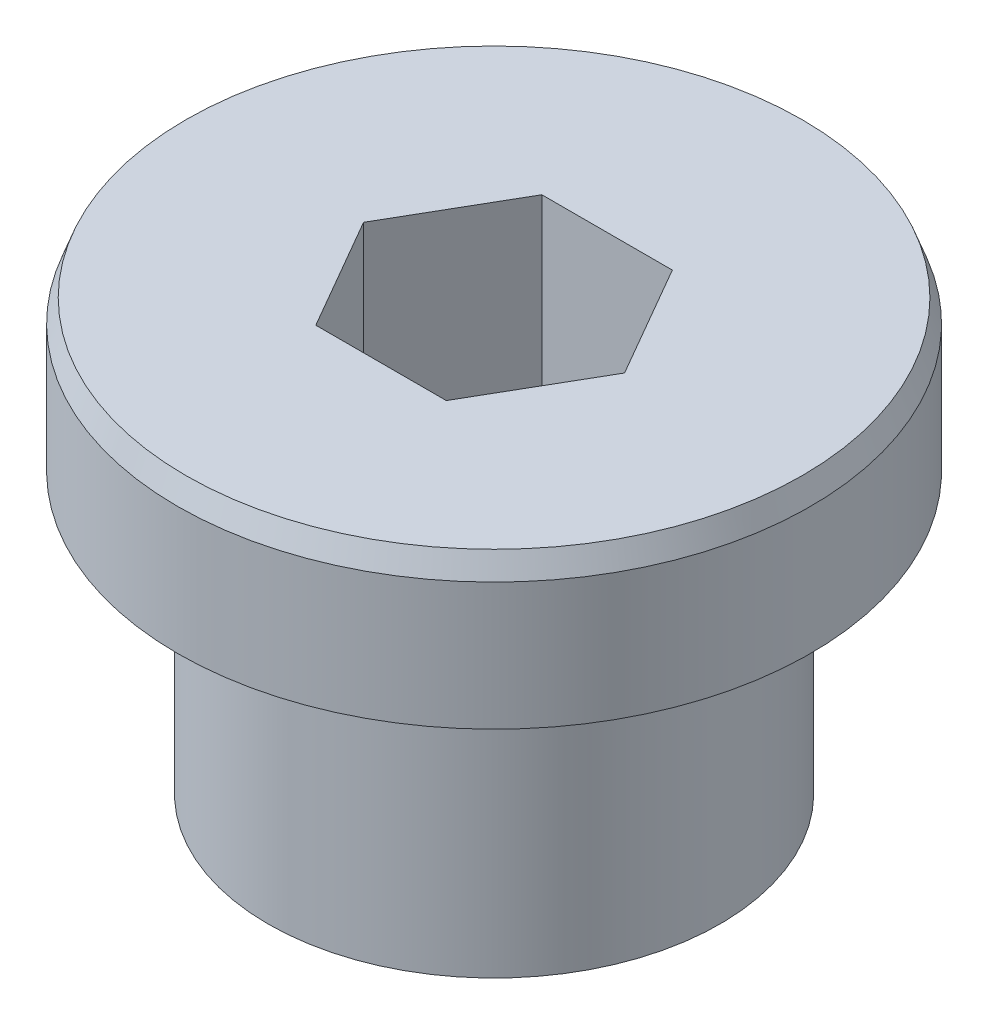
from build123d import *
from OCP.BRepFilletAPI import BRepFilletAPI_MakeChamfer

# Parameters (mm, degrees)
SKETCH1_R           = 5
BOSS_EXTRUDE1_DEPTH = 6
SKETCH3_R           = 7
BOSS_EXTRUDE2_DEPTH = 3.5
CUT_EXTRUDE1_DEPTH  = 5
CHAMFER1_SIZE       = 0.5
CHAMFER1_SIZE2      = 0.181985117


with BuildPart() as part:
    # Sketch1 → Boss-Extrude1 (new body)
    with BuildSketch(Plane(origin=(0, 0, 0), x_dir=(1, 0, 0), z_dir=(0, 1, 0))):
        with Locations(Location((0, 0, 0), (0, 0, 270))):
            Circle(SKETCH1_R)
    extrude(amount=BOSS_EXTRUDE1_DEPTH)

    # Sketch3 → Boss-Extrude2 (add)
    with BuildSketch(Plane(origin=(0, 6, 0), x_dir=(1, 0, 0), z_dir=(0, 1, 0))):
        with Locations(Location((0, 0, 0), (0, 0, 270))):
            Circle(SKETCH3_R)
    extrude(amount=BOSS_EXTRUDE2_DEPTH)

    # Sketch4 → Cut-Extrude1 (cut)
    with BuildSketch(Plane(origin=(0, 9.5, 0), x_dir=(1, 0, 0), z_dir=(0, 1, 0))):
        Polygon((-2.886751346, 0), (-1.443375673, -2.5), (1.443375673, -2.5), (2.886751346, 0), (1.443375673, 2.5), (-1.443375673, 2.5), align=None)
    extrude(amount=-CUT_EXTRUDE1_DEPTH, mode=Mode.SUBTRACT)

    # Chamfer1: one chamfer whose edges measure the first distance from different faces: ONE call of the kernel's chamfer builder (chamfer() names one face for all edges)
    chamfer1_edges_1 = [part.edges().sort_by_distance(p)[0] for p in [
        (0, 6, -7),
    ]]
    chamfer1_side_1 = [part.faces().sort_by_distance(p)[0] for p in [
        (0, 6, -6.802010101),
    ]]
    chamfer1_edges_2 = [part.edges().sort_by_distance(p)[0] for p in [
        (0, 9.5, -7),
    ]]
    chamfer1_side_2 = [part.faces().sort_by_distance(p)[0] for p in [
        (0, 7.75, -7),
    ]]
    chamfer1 = BRepFilletAPI_MakeChamfer(part.part.solid().wrapped)
    for e in chamfer1_edges_1:
        chamfer1.Add(CHAMFER1_SIZE, CHAMFER1_SIZE2, e.wrapped, chamfer1_side_1[0].wrapped)  # the first distance lies on this face
    for e in chamfer1_edges_2:
        chamfer1.Add(CHAMFER1_SIZE, CHAMFER1_SIZE2, e.wrapped, chamfer1_side_2[0].wrapped)  # the first distance lies on this face
    add(Compound.cast(chamfer1.Shape()), mode=Mode.REPLACE)


solid = part.part
